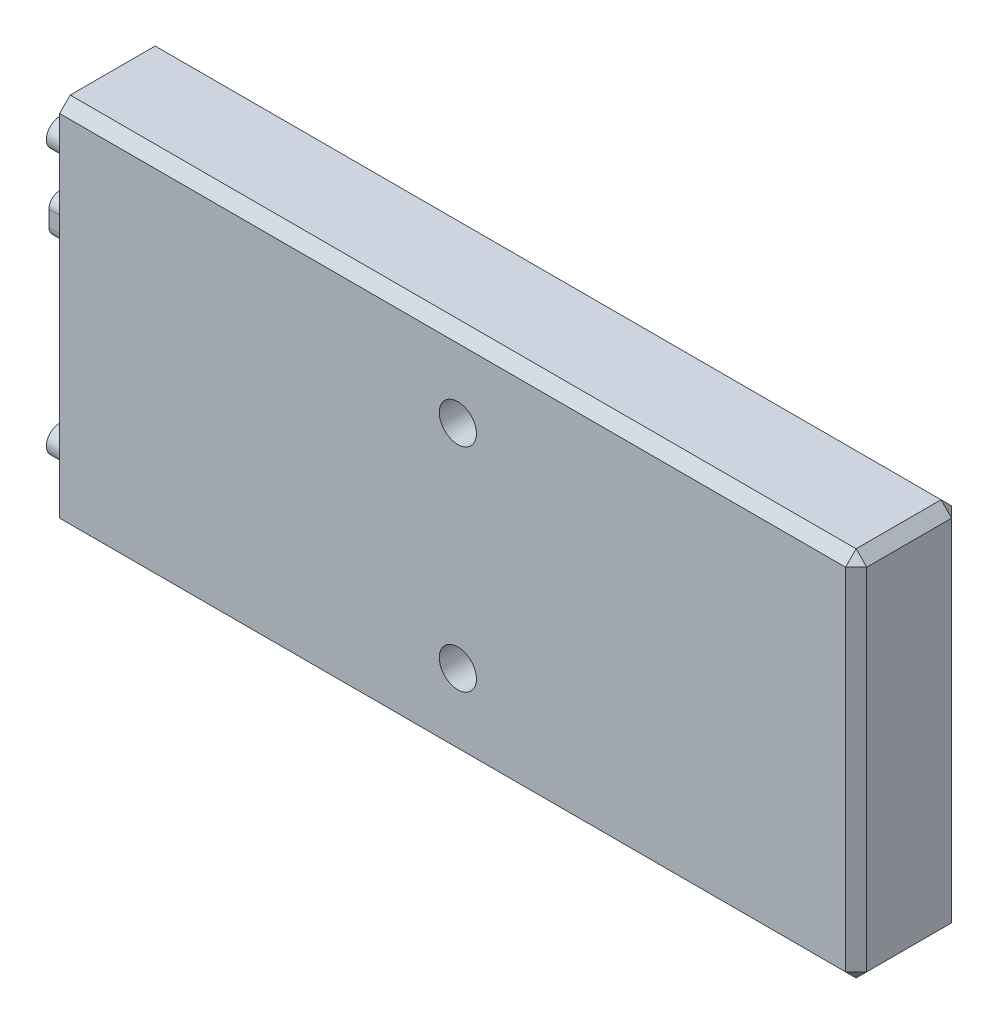
SolidWorks part; units mm, degrees
ref_plane "Front Plane" through (0, 0, 0) normal (0, 0, 1) x (1, 0, 0)
ref_plane "Top Plane" through (0, 0, 0) normal (0, 1, 0) x (1, 0, 0)
ref_plane "Right Plane" through (0, 0, 0) normal (1, 0, 0) x (0, 0, -1)
sketch "Sketch2" plane through (0, 0, 0) normal (0, 0, 1) x (1, 0, 0)
  line L1 (-75, 35) -> (75, 35)
  line L2 (-75, 35) -> (-75, -35)
  line L3 (-75, -35) -> (75, -35)
  line L4 (75, 35) -> (75, -35)
  line L5 (-75, 35) -> (75, -35) construction
  line L6 (-75, -35) -> (75, 35) construction
  point P0 (0, 0)
  dimension "D1" = 150
  dimension "D2" = 70
extrude "Boss-Extrude1" add sketch "Sketch2" along normal mid plane 20
sketch "Sketch3" plane through (-75, 0, 0) normal (-1, 0, 0) x (0, 0, 1)
  line L0 (10, -35) -> (-10, -35) construction
  line L1 (0, 0) -> (20.4786, 0) construction
  line L2 (5, 13.4136) -> (5, 10.4136) construction
  line L3 (7, 13.4136) -> (7, 10.4136)
  line L4 (3, 13.4136) -> (3, 10.4136)
  line L6 (-6.5, 15) -> (-3.5, 15)
  line L7 (-6.5, 15) -> (-6.5, 9)
  line L8 (-6.5, 9) -> (-3.5, 9)
  line L9 (-3.5, 15) -> (-3.5, 9)
  circle A0 centre (-5, -25) radius 2.5
  circle A1 centre (5, -25) radius 2.5
  circle A2 centre (-5, -25) radius 1
  circle A3 centre (5, -25) radius 1
  circle A4 centre (5, 25) radius 1
  circle A5 centre (5, 25) radius 2.5
  circle A6 centre (-5, 25) radius 2.5
  circle A7 centre (-5, 25) radius 1
  arc A8 (7, 13.4136) -> (3, 13.4136) centre (5, 13.4136) ccw
  arc A9 (3, 10.4136) -> (7, 10.4136) centre (5, 10.4136) ccw
  point P19 (5, 11.9136)
  dimension "D1" = 5
  dimension "D2" = 5
  dimension "D4" = 5
  dimension "D5" = 2
  dimension "D10" = 2
  dimension "D3" = 10
  dimension "D6" = 1.5
  dimension "D7" = 3
  dimension "D8" = 6
  dimension "D9" = 15
  dimension "D11" = 3
extrude "Boss-Extrude2" add sketch "Sketch3" along normal blind 5
chamfer "Chamfer1" distance 2 angle 45 9 edges at (0, 35, -10) (75, -35, 0) (75, 0, -10) (75, 35, 0) (0, 35, 10) (75, 0, 10) (0, -35, -10) (-75, -35, 0) (0, -35, 10)
sketch "Sketch4" plane through (0, 0, 10) normal (0, 0, 1) x (1, 0, 0)
  circle A0 centre (0, 20) radius 3.5
  circle A1 centre (0, -20) radius 3.5
  dimension "D1" = 20
  dimension "D2" = 20
  dimension "D3" = 7
extrude "Cut-Extrude1" cut sketch "Sketch4" against normal through all
